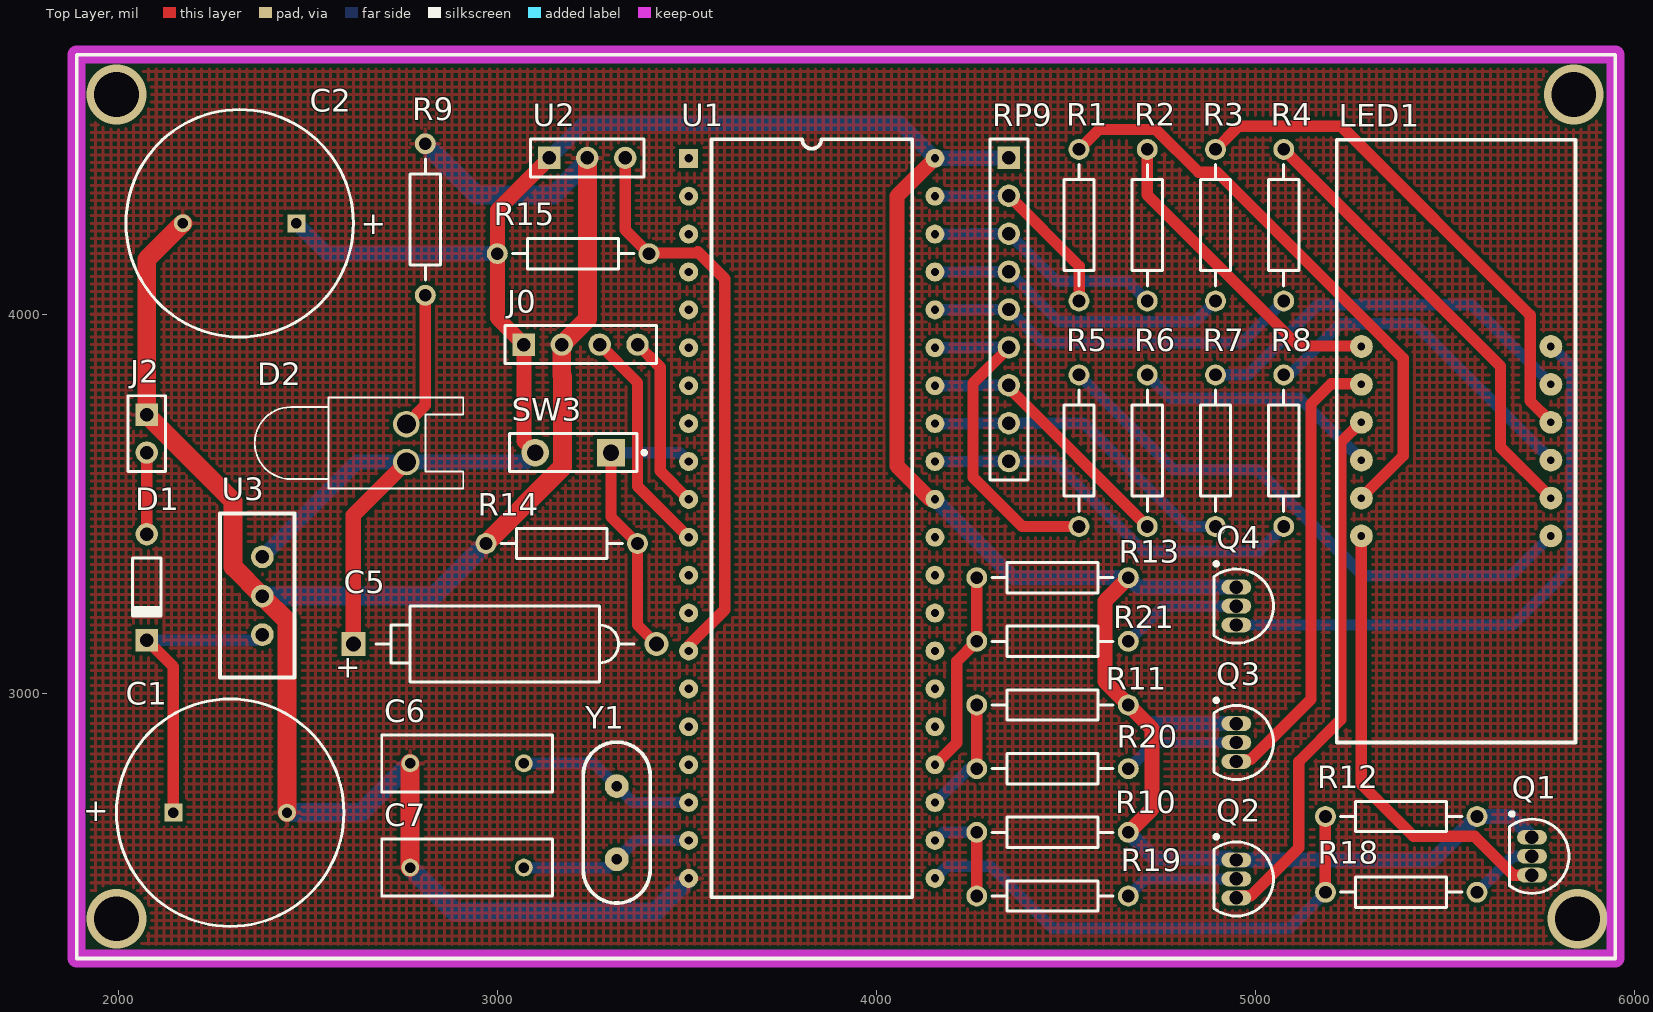
[diagram p0: Top Layer view]
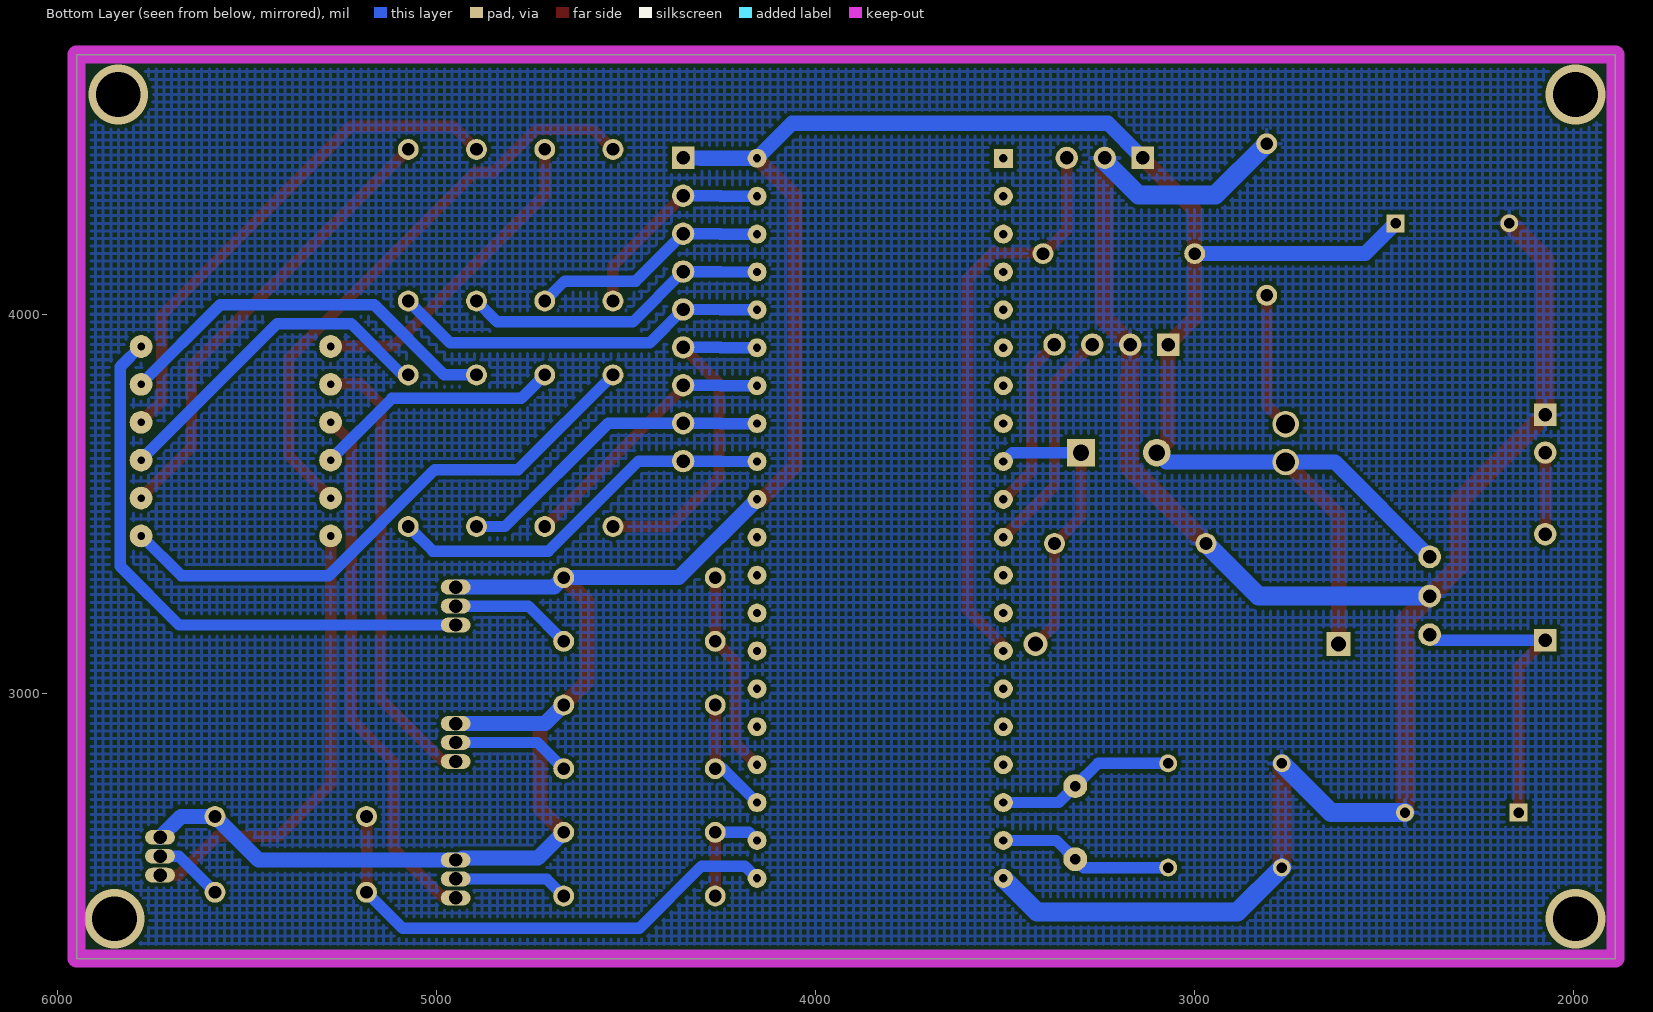
[diagram p1: Bottom Layer view, seen from below]
# Altium PCB MISC89328.PcbDoc
Units mil, origin at the board's own origin, x right, y up, seen from the top; angles counter-clockwise.
Board outline 4060 x 2385 mil, 2 copper layers (Top Layer, Bottom Layer); 39 components, 39 nets, 141 pads, 4 vias.

## Layer stack, top to bottom (the 12.6 mil dielectric is the usual default, probably not edited)
Top Solder: solder mask 0.4, Solder Resist, Dk 3.5
Top Layer: signal copper 1.4
Dielectric 1: dielectric 12.6, FR-4, Dk 4.8
Bottom Layer: signal copper 1.4
Bottom Solder: solder mask 0.4, Solder Resist, Dk 3.5

## Board outline
1890,2300 1890,4685 5950,4685 5950,2300

## Design rules (kind name [scope] priority, off if disabled: settings)
Clearance [All] p1: gap=10
HoleSize [All] p1: absolutevalues=TRUE maxlimit=500 minlimit=1 maxpercent=80.000 minpercent=20.000
MinimumSolderMaskSliver [All] p1: minsoldermaskwidth=2
PolygonConnect [All] p1: connectstyle=Relief reliefconductorwidth=10 reliefentries=4 polygonreliefangle="90 Angle" airgapwidth=10
RoomDefinition 频率测量电路 [InComponentClass('频率测量电路')] p1: confinementstyle=ConfineIn formatcopy=TRUE lockcomponents=FALSE outline 1890,2300 5945,2300 5945,4685 1890,4685
RoutingVias [All] p1: holewidth=28 width=50 viastyle="Through Hole" minholewidth=28 minwidth=50 maxholewidth=28 maxwidth=50
SilkToSilkClearance [All] p1: silktosilkclearance=2
SilkToSolderMaskClearance [IsPad] p1: minsilkscreentomaskgap=0 clearancetoexposedcopper=TRUE
SolderMaskExpansion [All] p1: expansion=4
Width GND [InNet('GND')] p1: maxlimit=55 minlimit=30 preferedwidth=50
Width VCC [InNet('5V')] p2: maxlimit=45 minlimit=30 preferedwidth=40
Width [All] p3: maxlimit=35 minlimit=20 preferedwidth=30
26 further rules are at their usual default settings.

## Components (designator, comment, footprint, x,y, rotation, side; value= is the part's Value field where it differs from the comment)
C1 "Cap Pol1" RB7.6-15 2295,2685 r180 top
C2 "Cap Pol1" RB7.6-15 2320,4240 r0 top
C5 "Cap Pol2" POLAR0.8 3020,3130 r180 top
C6 "Cap" RAD-0.3 2920,2815 r180 top
C7 "Cap" RAD-0.3 2920,2540 r180 top
D1 "Diode 1N914" DO-35 2075,3280 r270 top
D2 "LED0" LED-0 2760,3660 r270 top
J0 "Header 4" HDR1X4 3070,3920 r0 top
J2 "Header 2" HDR1X2 2075,3735 r270 top
LED1 "Dpy Red-CA" SIWEI 5844.96,2869.72 r90 top
Q1 "2N3906" TO-92A 5730,2570 r180 top
Q2 "2N3906" TO-92A 4950,2510 r180 top
Q3 "2N3906" TO-92A 4950,2870 r180 top
Q4 "2N3906" TO-92A 4950,3230 r180 top
R1 "Res2" AXIAL-0.4 4535,4235 r90 top
R2 "Res2" AXIAL-0.4 4715,4235 r90 top
R3 "Res2" AXIAL-0.4 4895,4235 r90 top
R4 "Res2" AXIAL-0.4 5075,4235 r90 top
R5 "Res2" AXIAL-0.4 4535,3640 r90 top
R6 "Res2" AXIAL-0.4 4715,3640 r90 top
R7 "Res2" AXIAL-0.4 4895,3640 r90 top
R8 "Res2" AXIAL-0.4 5075,3640 r90 top
R9 "Res2" AXIAL-0.4 2810,4250 r90 top
R10 "Res2" AXIAL-0.4 4465,2633 r180 top
R11 "Res2" AXIAL-0.4 4465,2969 r180 top
R12 "Res2" AXIAL-0.4 5385,2675 r180 top
R13 "Res2" AXIAL-0.4 4465,3305 r180 top
R14 "Res2" AXIAL-0.4 3170,3395 r180 top
R15 "Res2" AXIAL-0.4 3200,4160 r180 top
R18 "Res2" AXIAL-0.4 5385,2475 r180 top
R19 "Res2" AXIAL-0.4 4465,2465 r180 top
R20 "Res2" AXIAL-0.4 4465,2801 r180 top
R21 "Res2" AXIAL-0.4 4465,3137 r180 top
RP9 "20k" HDR1X9 4349.76,4412.62 r270 top
SW3 "SW-PB" SPST-2 3200,3635 r180 top
U1 "89c51" 89c51 3504.76,4411.56 r0 top
U2 "AH49E" HDR1X3 3137.39,4412.62 r0 top
U3 "7805" PCBComponent_1 2465,3041.5 r90 top
Y1 "Component_1" LC-HC-49S 3315,2658.54 r90 top

## Footprints (in the part's own frame and the unit in brackets; to place one, negate y for a bottom-side part, rotate by r counter-clockwise, add the part's x,y. Pads: shape width x height; smd on the part's side, far side on the other; paste and mask are expansions set on the pad)
89c51 [mil]
  rect 50x50 hole 22: 1(0,0)
  round 50 hole 22: 2(0,-100) 3(0,-200) 4(0,-300) 5(0,-400) 6(0,-500) 7(0,-600) 8(0,-700) 9(0,-800) 10(0,-900) 11(0,-1000) 12(0,-1100) 13(0,-1200) 14(0,-1300) 15(0,-1400) 16(0,-1500) 17(0,-1600) 18(0,-1700) 19(0,-1800) 20(0,-1900) 21(650,-1900) 22(650,-1800) 23(650,-1700) 24(650,-1600) 25(650,-1500) 26(650,-1400) 27(650,-1300) 28(650,-1200) 29(650,-1100) 30(650,-1000) 31(650,-900) 32(650,-800) 33(650,-700) 34(650,-600) 35(650,-500) 36(650,-400) 37(650,-300) 38(650,-200) 39(650,-100) 40(650,0)
  silkscreen extent 60,-1950 590,50, body extent 65,-1950 590,55, height 190
AXIAL-0.4 [mm] "Axial Device, Thru-Hole; 2 Leads; 0.4 in Pin Spacing"
  round 1.4 hole 0.85: 1(-5.08,0) 2(5.08,0)
  silkscreen extent -4.06,-1.02 4.06,1.02
DO-35 [mm] "Diode, Axial; Body 3.8 x 1.9 mm (LxDia. max), Lead Dia. 0.53 mm (max)"
  round 1.5 hole 0.9: 1(-3.55,0)
  rect 1.5x1.5 hole 0.9: 2(3.55,0)
  silkscreen extent -1.95,-0.95 2.05,0.95
HDR1X2 [mm] "Connector; Header; 2 Position"
  rect 1.5x1.5 hole 0.9: 1(0,0)
  round 1.5 hole 0.9: 2(2.54,0)
  silkscreen extent -1.27,-1.27 3.81,1.27
HDR1X3 [mm] "Connector; Header; 3 Position"
  rect 1.5x1.5 hole 0.9: 1(0,0)
  round 1.5 hole 0.9: 2(2.54,0) 3(5.08,0)
  silkscreen extent -1.27,-1.27 6.35,1.27
HDR1X4 [mm] "Connector; Header; 4 Position"
  rect 1.5x1.5 hole 0.9: 1(0,0)
  round 1.5 hole 0.9: 2(2.54,0) 3(5.08,0) 4(7.62,0)
  silkscreen extent -1.27,-1.27 8.89,1.27
HDR1X9 [mm] "Connector; Header; 9 Position"
  rect 1.5x1.5 hole 0.9: 1(0,0)
  round 1.5 hole 0.9: 2(2.54,0) 3(5.08,0) 4(7.62,0) 5(10.16,0) 6(12.7,0) 7(15.24,0) 8(17.78,0) 9(20.32,0)
  silkscreen extent -1.27,-1.27 21.59,1.27
LC-HC-49S [mm]
  round 1.6 hole 0.7: 1(-2.45,0) 2(2.45,0)
  silkscreen extent -5.39,-2.25 5.39,2.25, body extent -5.39,-2.27 5.41,2.23, height 3.6
LED-0 [mil] "LED; 2 Leads"
  round 70 hole 50: 1(50,0) 2(-50,0)
  silkscreen extent -120,-400 120,150
PCBComponent_1 [mil]
  round 60 hole 35.83: 1(113.03,85) 2(215,85) 3(318.5,85)
  silkscreen extent 0,0 433,197
POLAR0.8 [mm] "Polarized Capacitor; 2 Leads"
  rect 1.6x1.6 hole 1: 1(10.16,0)
  round 1.6 hole 1: 2(-10.16,0)
  silkscreen extent -8.64,-2.54 8.64,2.54
RAD-0.3 [mm] "Radial Cap, Thru-Hole; 2 Leads; 0.3 in Pin Spacing"
  round 1.2 hole 0.7: 1(-3.81,0) 2(3.81,0)
  silkscreen extent -5.71,-1.91 5.71,1.91
RB7.6-15 [mm] "Polarized Capacitor (Radial); 2 Leads"
  rect 1.2x1.2 hole 0.7: 1(3.81,0)
  round 1.2 hole 0.7: 2(-3.81,0)
  silkscreen extent -7.62,-7.62 7.62,7.62
SIWEI [mm]
  round 1.524 hole 0.51: 1(13.85,1.65) 2(16.39,1.65) 3(18.93,1.65) 4(21.47,1.65) 5(24.01,1.65) 6(26.55,1.65) 7(26.55,14.35) 8(24.01,14.35) 9(21.47,14.35) 10(18.93,14.35) 11(16.39,14.35) 12(13.85,14.35)
  silkscreen extent 0,0 40.4,16
SPST-2 [mm] "Switch; 2 Leads"
  rect 1.85x1.85 hole 1.1: 1(-2.54,0)
  round 1.85 hole 1.1: 2(2.54,0)
  silkscreen extent -4.89,-1.27 4.28,1.27
TO-92A [mm] "TO, Flat Index; 3 In-Line, Axial Leads; Body Dia. 4.5mm; Leads 0.51 x 0.48 mm (max)"
  oval 2x1 hole 0.9: 1(0,-1.27) 2(0,0) 3(0,1.27)
  silkscreen extent -2.48,-2.95 1.5,2.48, body extent -2.48,-2.5 1.5,2.5, height 6.86

## Part data
C1 C2: "Polarized Capacitor (Radial)"
C5: "Polarized Capacitor (Axial)"
C6 C7: "Capacitor"
D1: "High Conductance Fast Diode"
D2: "Typical INFRARED GaAs LED"
J0: "Header, 4-Pin"
J2: "Header, 2-Pin"
LED1: "7.62 mm Black Surface HER 7-Segment Display: CA, RH DP"
Q1 Q2 Q3 Q4: "PNP General Purpose Amplifier"
R1 R2 R3 R4 R5 R6 R7 R8 R9 R10 R11 R12 R13 R14 R15 R18 R19 R20 R21: "Resistor"
RP9: library part "Header 9", "Header, 9-Pin"
SW3: "Switch"
U1: library part Component_1
U2: library part "Header 3", "Header, 3-Pin"
U3: library part "Volt Reg", "Voltage Regulator"

## Via types
v1: diameter 157.48, hole 118.11, Top Layer to Bottom Layer, 4 vias

## Nets (pads, with @x,y where several pads share a name; then routed paths per layer and width w, separated by ;. In a path a pad name is that pad's centre, name@x,y a point inside that pad or via, vN(x,y) a via of type N, cw(c..) or ccw(c..) an arc to the next point about the centre after c; other vN are vias at no path point)
5V: C2.1 C5.1 D2.1 J0.1 Q1.1 Q2.1 Q3.1 Q4.1 R10.1 R11.1 R12.1 R13.1 R15.2 RP9.1 SW3.2 U1.31 U1.40 U2.1 U3.3 | length 8200.6
  Top Layer w40: C5.1 2620,3470 D2.1 ; SW3.2 3070,3665 J0.1 3000,3990 R15.2 3000,4275.24 U2.1 ; U1.31 4143.44,3511.56 4055,3600 4055,4311.8 U1.40 ; R10.1 4727,2695 4727,2907 R11.1 4603,3031 4603,3243 R13.1
  Bottom Layer w40: U3.3 2630,3610 D2.1 3075,3610 SW3.2 ; C2.1 2550,4160 R15.2@2995,4160 ; U2.1 3228.76,4504 4062.32,4504 U1.40 4303.88,4411.56 RP9.1 ; U1.31 4361.32,3305 R13.1 4690,3280 Q4.1 ; R10.1 4733,2565 Q2.1@4932,2565 ; R11.1 4714,2920 Q3.1 ; Q2.1 5470,2560 R12.1 5675,2675 Q1.1
COM1: LED1.12 Q1.3 | length 1205.7
  Top Layer w30: LED1.12@5280,3416.28 LED1.12 5280,2760 5417.56,2622.44 5578.56,2622.44 5681,2520 Q1.3
COM2: LED1.9 Q2.3 | length 1412.2
  Top Layer w30: Q2.3 4955.31,2465.32 4988.19,2465.32 5115,2592.12 5115,2820 5225,2930 5225,3661.28 LED1.9@5280,3716.28
COM3: LED1.8 Q3.3 | length 1199.1
  Top Layer w30: Q3.3 4955.31,2825.32 4988.19,2825.32 5147,2984.12 5147,3763.28 5200,3816.28 LED1.8@5280,3816.28
COM4: LED1.6 Q4.3 | length 1553.3
  Bottom Layer w30: Q4.3 5680,3180 5835,3335 5835,3861.28 LED1.6@5780,3916.28
GND: C1.2 C2.2 C6.2 C7.2 J0.2 J2.1 R9.2 R14.2 U1.20 U2.2 U3.2 | length 5527.5
  Top Layer w50: C2.2 2075,4145 J2.1 2303,3507 2303,3333.5 U3.2 2445,3191.5 C1.2 ; C7.2 C6.2 ; R14.2 3172,3597 3172,3836 3170,3838 J0.2 3237.39,3987.39 U2.2
  Bottom Layer w50: U3.2 2831.5,3256.5 R14.2 ; C1.2 2640,2685 C6.2 ; C7.2 2887,2423 3416.2,2423 U1.20 ; R9.2 2945,4315 3148.32,4315 3237.39,4404.07 U2.2
NetC1_1: C1.1 D1.2 U3.1 | length 795.2
  Top Layer w30: D1.2 2145,3070.24 C1.1
  Bottom Layer w30: D1.2 2365.71,3140.24 U3.1
NetC6_1: C6.1 U1.18 Y1.2 | length 477.6
  Bottom Layer w30: C6.1 3255,2815 Y1.2 3358.44,2711.56 U1.18
NetC7_1: C7.1 U1.19 Y1.1 | length 464.4
  Bottom Layer w30: C7.1 3292.91,2540 Y1.1 3364.47,2611.56 U1.19
NetD1_1: D1.1 J2.2 | length 215.2
  Top Layer w30: D1.1 J2.2
NetD2_2: D2.2 R9.1 | length 360.7
  Top Layer w30: D2.2 2810,3760 R9.1
NetLED1_1: LED1.1 R5.2 | length 1508.6
  Bottom Layer w30: R5.2 4785,3590 5005,3590 5285,3310 5673.72,3310 LED1.1@5780,3416.28
NetLED1_2: LED1.2 R4.2 | length 1210.7
  Top Layer w30: R4.2 5647,3863 5647,3649.28 LED1.2@5780,3516.28
NetLED1_3: LED1.3 R8.2 | length 909.5
  Bottom Layer w30: R8.2 5090,3840 5225,3975 5421.28,3975 LED1.3@5780,3616.28
NetLED1_4: LED1.4 R3.2 | length 1366
  Top Layer w30: R3.2 4956,4496 5227,4496 5725,3998 5725,3771.28 LED1.4@5780,3716.28
NetLED1_5: LED1.5 R7.2 | length 1048.1
  Bottom Layer w30: R7.2 4980,3840 5165,4025 5571.28,4025 LED1.5@5780,3816.28
NetLED1_7: LED1.7 R2.2 | length 850.2
  Top Layer w30: R2.2 4715,4315 5113.72,3916.28 LED1.7@5280,3916.28
NetLED1_10: LED1.10 R6.2 | length 657.7
  Bottom Layer w30: R6.2 4777,3778 5118.28,3778 LED1.10@5280,3616.28
NetLED1_11: LED1.11 R1.2 | length 1540.1
  Top Layer w30: R1.2 4587.56,4487.56 4737.44,4487.56 4850,4375 4899.07,4375 5302.78,3971.28 5390,3884.07 5390,3626.28 LED1.11@5280,3516.28
NetQ1_2: Q1.2 R18.1 | length 184.4
  Bottom Layer w30: R18.1 5680,2570 Q1.2
NetQ2_2: Q2.2 R19.1 | length 303.6
  Bottom Layer w30: R19.1 4710,2510 Q2.2
NetQ3_2: Q3.2 R20.1 | length 313.6
  Bottom Layer w30: R20.1 4734,2870 Q3.2
NetQ4_2: Q4.2 R21.1 | length 323.5
  Bottom Layer w30: R21.1 4758,3230 Q4.2
P0.0: R1.1 RP9.2 U1.39 | length 549.8
  Top Layer w30: RP9.2 4535,4127.39 R1.1
  Bottom Layer w30: U1.39 4251,4311.56 4252.06,4312.62 RP9.2
P0.1: R2.1 RP9.3 U1.38 | length 634.2
  Bottom Layer w30: U1.38 4251,4211.56 4252.06,4212.62 RP9.3 4474.83,4087.56 4662.44,4087.56 R2.1
P0.2: R3.1 RP9.4 U1.37 | length 818.4
  Bottom Layer w30: U1.37 4251,4111.56 4252.06,4112.62 RP9.4 4482.39,3980 4840,3980 R3.1
P0.3: R4.1 RP9.5 U1.36 | length 1002.5
  Bottom Layer w30: U1.36 4251,4011.56 4252.06,4012.62 RP9.5 4437.39,3925 4965,3925 R4.1
P0.4: R5.1 RP9.6 U1.35 | length 911.2
  Top Layer w30: RP9.6 4255,3817.86 4255,3570 4385,3440 R5.1
  Bottom Layer w30: U1.35 4251,3911.56 4252.06,3912.62 RP9.6
P0.5: R6.1 RP9.7 U1.34 | length 719.3
  Top Layer w30: RP9.7 4349.76,3805.24 R6.1
  Bottom Layer w30: U1.34 4251,3811.56 4252.06,3812.62 RP9.7
P0.6: R7.1 RP9.8 U1.33 | length 853.6
  Bottom Layer w30: U1.33 4251,3711.56 4252.06,3712.62 RP9.8 4547.38,3712.62 4820,3440 R7.1
P0.7: R8.1 RP9.9 U1.32 | length 1046
  Bottom Layer w30: U1.32 4251,3611.56 4252.06,3612.62 RP9.9 4467.38,3612.62 4705,3375 5010,3375 R8.1
P2.0: R12.2 R18.2 U1.21 | length 1351
  Top Layer w30: R18.2 R12.2
  Bottom Layer w30: U1.21 4187.2,2544 4301,2544 4465,2380 5090,2380 R18.2
P2.1: R10.2 R19.2 U1.22 | length 287.1
  Top Layer w30: R19.2 R10.2
  Bottom Layer w30: U1.22 4176.2,2633 R10.2
P2.2: R11.2 R20.2 U1.23 | length 315.3
  Top Layer w30: R20.2 R11.2
  Bottom Layer w30: U1.23 4244.2,2801 R20.2
P2.3: R13.2 R21.2 U1.24 | length 539.1
  Top Layer w30: U1.24 4212,2868.8 4212,3084 R21.2 R13.2
P3.4: R15.1 U1.14 U2.3 | length 1530.6
  Top Layer w30: U2.3 3337.39,4222.61 3398.44,4161.56 3525.47,4161.56 3528.91,4165 3600,4093.91 3600,3220.37 3504.76,3125.13 U1.14
REST: C5.2 R14.1 SW3.1 U1.9 | length 769.2
  Top Layer w30: SW3.1 3300,3465 R14.1 3370,3180 C5.2
  Bottom Layer w30: SW3.1 3481.32,3635 U1.9
RXD: J0.4 U1.10 | length 464.3
  Top Layer w30: J0.4 3430,3860 3430,3586.32 U1.10
TXD: J0.3 U1.11 | length 605.7
  Top Layer w30: J0.3 3370,3820 3370,3546.32 U1.11
pads on no net: U1.1 U1.2 U1.3 U1.4 U1.5 U1.6 U1.7 U1.8 U1.12 U1.13 U1.15 U1.16 U1.17 U1.25 U1.26 U1.27 U1.28 U1.29 U1.30
copper on no net:
  other v1: 1995,2405 5850,2405 1995,4580 5840,4580

## Polygon pours and split planes (outlines as drawn)
GND on Top Layer "Top Layer-No Net" (hatched 90Degree grid 20 track 8, pour order 6): 1890,4685 5950,4685 5950,2310 5940,2300 1890,2300
GND on Bottom Layer "Top Layer-No Net" (hatched 90Degree grid 20 track 8, pour order 8): 1910,4685 5940,4685 5950,4675 5950,2330 1940,2330 1910,2300

## Keep-outs
Keep-Out Layer:
  the board outline again, w47.24

## Silkscreen, mask and mechanical layers (free items; w line width, h text height)
Top Overlay:
  the board outline again, w10